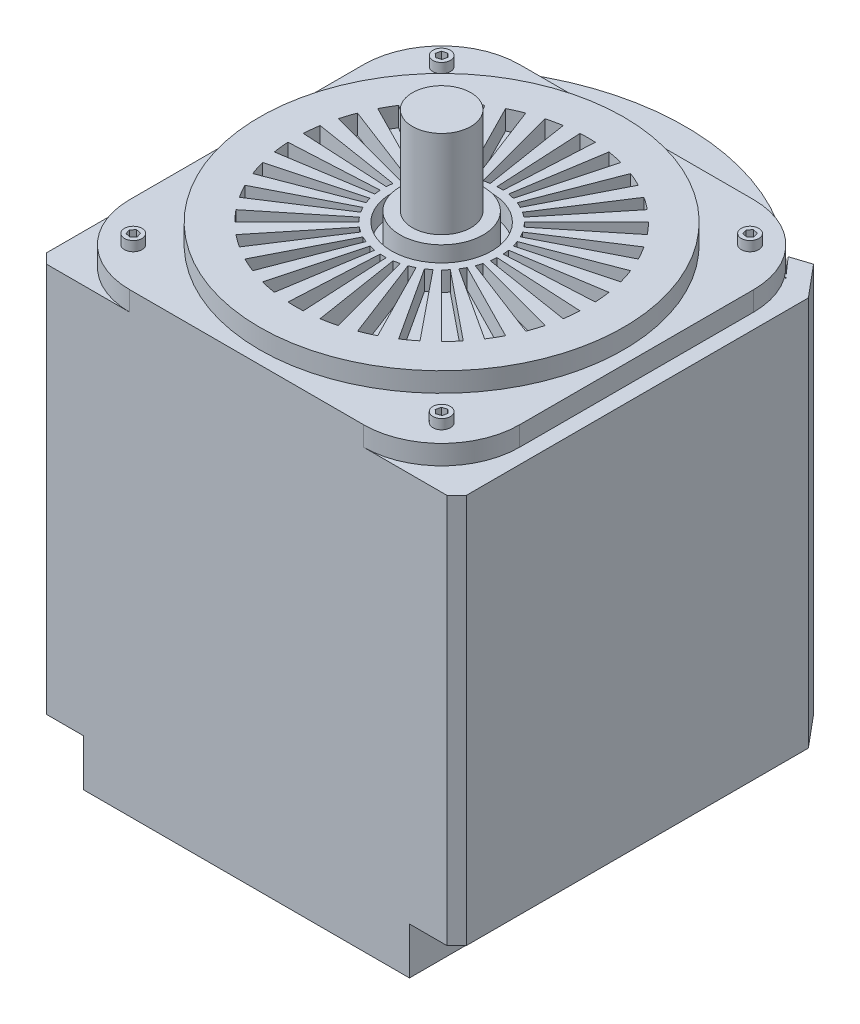
from build123d import *

# Parameters (mm, degrees)
BOSS_EXTRUDE1_DEPTH  = 200
BOSS_EXTRUDE2_DEPTH  = 200
BOSS_EXTRUDE5_DEPTH  = 10
SKETCH4_W            = 215.39447181
SKETCH4_H            = 200
BOSS_EXTRUDE6_DEPTH  = 17.479413836
BOSS_EXTRUDE7_START  = -30
BOSS_EXTRUDE7_DEPTH  = 30
SKETCH6_R            = 93.394786631
SKETCH6_R_2          = 25.673821091
BOSS_EXTRUDE8_DEPTH  = 10
SKETCH7_R            = 21.331945156
BOSS_EXTRUDE9_DEPTH  = 15
SKETCH8_R            = 15
BOSS_EXTRUDE10_DEPTH = 45
SKETCH9_R            = 4.5
BOSS_EXTRUDE11_DEPTH = 5
CUT_EXTRUDE1_DEPTH   = 4
CIRPATTERN1_COUNT    = 4
BOSS_EXTRUDE12_DEPTH = 4
BOSS_EXTRUDE13_DEPTH = 24
CHAMFER1_SIZE        = 5
SKETCH13_R           = 6.5
CUT_EXTRUDE2_DEPTH   = 30
SKETCH14_R           = 5.5
BOSS_EXTRUDE14_DEPTH = 4


with BuildPart() as part:
    # Sketch1 → Boss-Extrude1 (new body)
    with BuildSketch(Plane(origin=(0, 0, 0), x_dir=(1, 0, 0), z_dir=(0, 1, 0))):
        with BuildLine():
            Line((-1.5, 124.990999676), (-5.554426032, 109.85967573))
            ThreePointArc((-5.554426032, 109.85967573), (-7.673212112, 109.732045529), (-9.789141002, 109.563555612))
            Line((-9.789141002, 109.563555612), (-15.909982914, 123.983355511))
            ThreePointArc((-15.909982914, 123.983355511), (-17.39663762, 123.783508593), (-18.88078712, 123.565836208))
            Line((-18.88078712, 123.565836208), (-20.789882481, 108.017502223))
            ThreePointArc((-20.789882481, 108.017502223), (-22.87028599, 107.596236081), (-24.942173542, 107.134905512))
            Line((-24.942173542, 107.134905512), (-33.010296108, 120.562516359))
            ThreePointArc((-33.010296108, 120.562516359), (-34.454669477, 120.157711992), (-35.894081196, 119.735604292))
            Line((-35.894081196, 119.735604292), (-35.620687516, 104.072890903))
            ThreePointArc((-35.620687516, 104.072890903), (-37.622215766, 103.366188286), (-39.609735045, 102.620996339))
            Line((-39.609735045, 102.620996339), (-49.468101436, 114.795064965))
            ThreePointArc((-49.468101436, 114.795064965), (-50.842080384, 114.193182205), (-52.208737809, 113.574855036))
            Line((-52.208737809, 113.574855036), (-49.758176387, 98.102619143))
            ThreePointArc((-49.758176387, 98.102619143), (-51.641871906, 97.124235214), (-53.50633811, 96.109686203))
            Line((-53.50633811, 96.109686203), (-64.96306644, 106.793258208))
            ThreePointArc((-64.96306644, 106.793258208), (-66.239908029, 106.00601202), (-67.507210728, 105.203500416))
            Line((-67.507210728, 105.203500416), (-62.927178953, 90.222891491))
            ThreePointArc((-62.927178953, 90.222891491), (-64.656377752, 88.991869381), (-66.361501167, 87.727710348))
            Line((-66.361501167, 87.727710348), (-79.193599249, 96.712842156))
            ThreePointArc((-79.193599249, 96.712842156), (-80.348451211, 95.75555539), (-81.491732579, 94.784479327))
            Line((-81.491732579, 94.784479327), (-74.87137556, 80.587077884))
            ThreePointArc((-74.87137556, 80.587077884), (-76.41242075, 79.127378037), (-77.925013089, 77.638214399))
            Line((-77.925013089, 77.638214399), (-91.882718731, 84.750020641))
            ThreePointArc((-91.882718731, 84.750020641), (-92.893103185, 83.641325795), (-93.89011055, 82.520586164))
            Line((-93.89011055, 82.520586164), (-93.89011055, -82.520586164))
            Line((-93.89011055, -82.520586164), (93.697235905, -82.520586164))
            Line((93.697235905, -82.520586164), (93.697235905, 82.739518876))
            ThreePointArc((93.697235905, 82.739518876), (92.697615235, 83.857928247), (91.684645627, 84.964261641))
            Line((91.684645627, 84.964261641), (77.743578328, 77.819894814))
            ThreePointArc((77.743578328, 77.819894814), (76.24293888, 79.290694731), (74.714479133, 80.732562253))
            Line((74.714479133, 80.732562253), (81.307207406, 94.942814493))
            ThreePointArc((81.307207406, 94.942814493), (80.162039302, 95.911664853), (79.005327449, 96.866703436))
            Line((79.005327449, 96.866703436), (66.190731164, 87.856628139))
            ThreePointArc((66.190731164, 87.856628139), (64.50048555, 89.104923342), (62.786704343, 90.320705034))
            Line((62.786704343, 90.320705034), (67.343418819, 105.308422939))
            ThreePointArc((67.343418819, 105.308422939), (66.074868843, 106.108961485), (64.796803743, 106.894219791))
            Line((64.796803743, 106.894219791), (53.356714297, 96.192832578))
            ThreePointArc((53.356714297, 96.192832578), (51.509578449, 97.194461406), (49.643647261, 98.16062493))
            Line((49.643647261, 98.16062493), (52.07614942, 113.635710327))
            ThreePointArc((52.07614942, 113.635710327), (50.708771279, 114.252442054), (49.334090811, 114.852720838))
            Line((49.334090811, 114.852720838), (39.489939448, 102.667154837))
            ThreePointArc((39.489939448, 102.667154837), (37.521666022, 103.402730036), (35.53970131, 104.100574594))
            Line((35.53970131, 104.100574594), (35.800908304, 119.76349596))
            ThreePointArc((35.800908304, 119.76349596), (34.361168595, 120.184483578), (32.916480699, 120.588164006))
            Line((32.916480699, 120.588164006), (24.858808122, 107.154279703))
            ThreePointArc((24.858808122, 107.154279703), (22.807494482, 107.60956368), (20.747858611, 108.025581984))
            Line((20.747858611, 108.025581984), (18.832714591, 123.573172093))
            ThreePointArc((18.832714591, 123.573172093), (17.348480521, 123.790267079), (15.861748181, 123.989535626))
            Line((15.861748181, 123.989535626), (9.7465165, 109.567355613))
            ThreePointArc((9.7465165, 109.567355613), (7.651867312, 109.733536016), (5.554426032, 109.85967573))
            Line((5.554426032, 109.85967573), (1.5, 124.990999676))
            ThreePointArc((1.5, 124.990999676), (0, 125), (-1.5, 124.990999676))
        make_face()
    extrude(amount=BOSS_EXTRUDE1_DEPTH)

    # Sketch2 → Boss-Extrude2 (add)
    with BuildSketch(Plane(origin=(0, 200, 0), x_dir=(1, 0, 0), z_dir=(0, 1, 0))):
        Polygon((-93.89011055, 82.520586164), (-84.247016889, 93.492286342), (-94.044433488, 96.7026075), (-107.697235905, 80.401462252), (-107.697235905, -82.520586164), (-93.89011055, -82.520586164), align=None)
        Polygon((93.697235905, 82.739518876), (93.697235905, -82.520586164), (107.697235905, -82.520586164), (107.697235905, 80.401462252), (94.044433488, 96.7026075), (84.247016889, 93.492286342), align=None)
    extrude(amount=-BOSS_EXTRUDE2_DEPTH)

    # Sketch3 → Boss-Extrude5 (add)
    with BuildSketch(Plane(origin=(0, 200, 0), x_dir=(1, 0, 0), z_dir=(0, 1, 0))):
        with BuildLine():
            Line((-60, -100), (60, -100))
            ThreePointArc((60, -100), (88.284271247, -88.284271247), (100, -60))
            Line((100, -60), (100, 60))
            ThreePointArc((100, 60), (88.284271247, 88.284271247), (60, 100))
            Line((60, 100), (-60, 100))
            ThreePointArc((-60, 100), (-88.284271247, 88.284271247), (-100, 60))
            Line((-100, 60), (-100, -60))
            ThreePointArc((-100, -60), (-88.284271247, -88.284271247), (-60, -100))
        make_face()
    extrude(amount=BOSS_EXTRUDE5_DEPTH)

    # Sketch4 → Boss-Extrude6 (add)
    with BuildSketch(Plane.XY.offset(82.520586164)):
        with Locations((0, 100)):
            Rectangle(SKETCH4_W, SKETCH4_H)
    extrude(amount=BOSS_EXTRUDE6_DEPTH)

    # Sketch5 → Boss-Extrude7 (add)
    with BuildSketch(Plane(origin=(0, 200, 0), x_dir=(1, 0, 0), z_dir=(0, 1, 0)).offset(BOSS_EXTRUDE7_START)):
        with BuildLine():
            Line((-102.459320776, 71.603684167), (0, 0))
            Line((0, 0), (95.193765048, 81.013252595))
            ThreePointArc((95.193765048, 81.013252595), (-5.944078525, 124.858591737), (-102.459320776, 71.603684167))
        make_face()
    boss_extrude7 = extrude(amount=BOSS_EXTRUDE7_DEPTH)

    # Mirror2: Boss-Extrude7 across plane
    add(boss_extrude7.mirror(Plane(origin=(0, 100, 0), x_dir=(0, 0, 1), z_dir=(0, -1, 0))))

    # Sketch6 → Boss-Extrude8 (add)
    with BuildSketch(Plane(origin=(0, 210, 0), x_dir=(1, 0, 0), z_dir=(0, 1, 0))):
        with Locations(Location((0, 0, 0), (0, 0, 270))):
            Circle(SKETCH6_R)
        with Locations(Location((0, 0, 0), (0, 0, 270))):
            Circle(SKETCH6_R_2, mode=Mode.SUBTRACT)
        with BuildLine():
            Line((-3.925196718, 74.897215107), (-1.570078687, 29.958886043))
            ThreePointArc((-1.570078687, 29.958886043), (0, 30), (1.570078687, 29.958886043))
            Line((1.570078687, 29.958886043), (3.925196718, 74.897215107))
            ThreePointArc((3.925196718, 74.897215107), (0, 75), (-3.925196718, 74.897215107))
        make_face(mode=Mode.SUBTRACT)
        with BuildLine():
            Line((11.732584878, 74.076625545), (4.693033951, 29.630650218))
            ThreePointArc((4.693033951, 29.630650218), (6.237350725, 29.344428022), (7.764571353, 28.977774789))
            Line((7.764571353, 28.977774789), (19.411428383, 72.444436972))
            ThreePointArc((19.411428383, 72.444436972), (15.593376811, 73.361070055), (11.732584878, 74.076625545))
        make_face(mode=Mode.SUBTRACT)
        with BuildLine():
            Line((26.877596216, 70.018531987), (10.751038486, 28.007412795))
            ThreePointArc((10.751038486, 28.007412795), (12.202099292, 27.406363729), (13.619714992, 26.730195726))
            Line((13.619714992, 26.730195726), (34.04928748, 66.825489314))
            ThreePointArc((34.04928748, 66.825489314), (30.505248231, 68.515909323), (26.877596216, 70.018531987))
        make_face(mode=Mode.SUBTRACT)
        with BuildLine():
            Line((40.847927626, 62.900292596), (16.33917105, 25.160117038))
            ThreePointArc((16.33917105, 25.160117038), (17.633557569, 24.270509831), (18.879611731, 23.314378844))
            Line((18.879611731, 23.314378844), (47.199029329, 58.285947109))
            ThreePointArc((47.199029329, 58.285947109), (44.083893922, 60.676274578), (40.847927626, 62.900292596))
        make_face(mode=Mode.SUBTRACT)
        with BuildLine():
            Line((53.033008589, 53.033008589), (21.213203436, 21.213203436))
            ThreePointArc((21.213203436, 21.213203436), (22.294344764, 20.073918191), (23.314378844, 18.879611731))
            Line((23.314378844, 18.879611731), (58.285947109, 47.199029329))
            ThreePointArc((58.285947109, 47.199029329), (55.735861911, 50.184795477), (53.033008589, 53.033008589))
        make_face(mode=Mode.SUBTRACT)
        with BuildLine():
            Line((62.900292596, 40.847927626), (25.160117038, 16.33917105))
            ThreePointArc((25.160117038, 16.33917105), (25.980762114, 15), (26.730195726, 13.619714992))
            Line((26.730195726, 13.619714992), (66.825489314, 34.04928748))
            ThreePointArc((66.825489314, 34.04928748), (64.951905284, 37.5), (62.900292596, 40.847927626))
        make_face(mode=Mode.SUBTRACT)
        with BuildLine():
            Line((70.018531987, 26.877596216), (28.007412795, 10.751038486))
            ThreePointArc((28.007412795, 10.751038486), (28.531695489, 9.270509831), (28.977774789, 7.764571353))
            Line((28.977774789, 7.764571353), (72.444436972, 19.411428383))
            ThreePointArc((72.444436972, 19.411428383), (71.329238722, 23.176274578), (70.018531987, 26.877596216))
        make_face(mode=Mode.SUBTRACT)
        with BuildLine():
            Line((74.076625545, 11.732584878), (29.630650218, 4.693033951))
            ThreePointArc((29.630650218, 4.693033951), (29.835656861, 3.135853898), (29.958886043, 1.570078687))
            Line((29.958886043, 1.570078687), (74.897215107, 3.925196718))
            ThreePointArc((74.897215107, 3.925196718), (74.589142153, 7.839634745), (74.076625545, 11.732584878))
        make_face(mode=Mode.SUBTRACT)
        with BuildLine():
            Line((74.897215107, -3.925196718), (29.958886043, -1.570078687))
            ThreePointArc((29.958886043, -1.570078687), (29.835656861, -3.135853898), (29.630650218, -4.693033951))
            Line((29.630650218, -4.693033951), (74.076625545, -11.732584878))
            ThreePointArc((74.076625545, -11.732584878), (74.589142153, -7.839634745), (74.897215107, -3.925196718))
        make_face(mode=Mode.SUBTRACT)
        with BuildLine():
            Line((72.444436972, -19.411428383), (28.977774789, -7.764571353))
            ThreePointArc((28.977774789, -7.764571353), (28.531695489, -9.270509831), (28.007412795, -10.751038486))
            Line((28.007412795, -10.751038486), (70.018531987, -26.877596216))
            ThreePointArc((70.018531987, -26.877596216), (71.329238722, -23.176274578), (72.444436972, -19.411428383))
        make_face(mode=Mode.SUBTRACT)
        with BuildLine():
            Line((66.825489314, -34.04928748), (26.730195726, -13.619714992))
            ThreePointArc((26.730195726, -13.619714992), (25.980762114, -15), (25.160117038, -16.33917105))
            Line((25.160117038, -16.33917105), (62.900292596, -40.847927626))
            ThreePointArc((62.900292596, -40.847927626), (64.951905284, -37.5), (66.825489314, -34.04928748))
        make_face(mode=Mode.SUBTRACT)
        with BuildLine():
            Line((58.285947109, -47.199029329), (23.314378844, -18.879611731))
            ThreePointArc((23.314378844, -18.879611731), (22.294344764, -20.073918191), (21.213203436, -21.213203436))
            Line((21.213203436, -21.213203436), (53.033008589, -53.033008589))
            ThreePointArc((53.033008589, -53.033008589), (55.735861911, -50.184795477), (58.285947109, -47.199029329))
        make_face(mode=Mode.SUBTRACT)
        with BuildLine():
            Line((47.199029329, -58.285947109), (18.879611731, -23.314378844))
            ThreePointArc((18.879611731, -23.314378844), (17.633557569, -24.270509831), (16.33917105, -25.160117038))
            Line((16.33917105, -25.160117038), (40.847927626, -62.900292596))
            ThreePointArc((40.847927626, -62.900292596), (44.083893922, -60.676274578), (47.199029329, -58.285947109))
        make_face(mode=Mode.SUBTRACT)
        with BuildLine():
            Line((34.04928748, -66.825489314), (13.619714992, -26.730195726))
            ThreePointArc((13.619714992, -26.730195726), (12.202099292, -27.406363729), (10.751038486, -28.007412795))
            Line((10.751038486, -28.007412795), (26.877596216, -70.018531987))
            ThreePointArc((26.877596216, -70.018531987), (30.505248231, -68.515909323), (34.04928748, -66.825489314))
        make_face(mode=Mode.SUBTRACT)
        with BuildLine():
            Line((19.411428383, -72.444436972), (7.764571353, -28.977774789))
            ThreePointArc((7.764571353, -28.977774789), (6.237350725, -29.344428022), (4.693033951, -29.630650218))
            Line((4.693033951, -29.630650218), (11.732584878, -74.076625545))
            ThreePointArc((11.732584878, -74.076625545), (15.593376811, -73.361070055), (19.411428383, -72.444436972))
        make_face(mode=Mode.SUBTRACT)
        with BuildLine():
            Line((3.925196718, -74.897215107), (1.570078687, -29.958886043))
            ThreePointArc((1.570078687, -29.958886043), (0, -30), (-1.570078687, -29.958886043))
            Line((-1.570078687, -29.958886043), (-3.925196718, -74.897215107))
            ThreePointArc((-3.925196718, -74.897215107), (0, -75), (3.925196718, -74.897215107))
        make_face(mode=Mode.SUBTRACT)
        with BuildLine():
            Line((-11.732584878, -74.076625545), (-4.693033951, -29.630650218))
            ThreePointArc((-4.693033951, -29.630650218), (-6.237350725, -29.344428022), (-7.764571353, -28.977774789))
            Line((-7.764571353, -28.977774789), (-19.411428383, -72.444436972))
            ThreePointArc((-19.411428383, -72.444436972), (-15.593376811, -73.361070055), (-11.732584878, -74.076625545))
        make_face(mode=Mode.SUBTRACT)
        with BuildLine():
            Line((-26.877596216, -70.018531987), (-10.751038486, -28.007412795))
            ThreePointArc((-10.751038486, -28.007412795), (-12.202099292, -27.406363729), (-13.619714992, -26.730195726))
            Line((-13.619714992, -26.730195726), (-34.04928748, -66.825489314))
            ThreePointArc((-34.04928748, -66.825489314), (-30.505248231, -68.515909323), (-26.877596216, -70.018531987))
        make_face(mode=Mode.SUBTRACT)
        with BuildLine():
            Line((-40.847927626, -62.900292596), (-16.33917105, -25.160117038))
            ThreePointArc((-16.33917105, -25.160117038), (-17.633557569, -24.270509831), (-18.879611731, -23.314378844))
            Line((-18.879611731, -23.314378844), (-47.199029329, -58.285947109))
            ThreePointArc((-47.199029329, -58.285947109), (-44.083893922, -60.676274578), (-40.847927626, -62.900292596))
        make_face(mode=Mode.SUBTRACT)
        with BuildLine():
            Line((-53.033008589, -53.033008589), (-21.213203436, -21.213203436))
            ThreePointArc((-21.213203436, -21.213203436), (-22.294344764, -20.073918191), (-23.314378844, -18.879611731))
            Line((-23.314378844, -18.879611731), (-58.285947109, -47.199029329))
            ThreePointArc((-58.285947109, -47.199029329), (-55.735861911, -50.184795477), (-53.033008589, -53.033008589))
        make_face(mode=Mode.SUBTRACT)
        with BuildLine():
            Line((-62.900292596, -40.847927626), (-25.160117038, -16.33917105))
            ThreePointArc((-25.160117038, -16.33917105), (-25.980762114, -15), (-26.730195726, -13.619714992))
            Line((-26.730195726, -13.619714992), (-66.825489314, -34.04928748))
            ThreePointArc((-66.825489314, -34.04928748), (-64.951905284, -37.5), (-62.900292596, -40.847927626))
        make_face(mode=Mode.SUBTRACT)
        with BuildLine():
            Line((-70.018531987, -26.877596216), (-28.007412795, -10.751038486))
            ThreePointArc((-28.007412795, -10.751038486), (-28.531695489, -9.270509831), (-28.977774789, -7.764571353))
            Line((-28.977774789, -7.764571353), (-72.444436972, -19.411428383))
            ThreePointArc((-72.444436972, -19.411428383), (-71.329238722, -23.176274578), (-70.018531987, -26.877596216))
        make_face(mode=Mode.SUBTRACT)
        with BuildLine():
            Line((-74.076625545, -11.732584878), (-29.630650218, -4.693033951))
            ThreePointArc((-29.630650218, -4.693033951), (-29.835656861, -3.135853898), (-29.958886043, -1.570078687))
            Line((-29.958886043, -1.570078687), (-74.897215107, -3.925196718))
            ThreePointArc((-74.897215107, -3.925196718), (-74.589142153, -7.839634745), (-74.076625545, -11.732584878))
        make_face(mode=Mode.SUBTRACT)
        with BuildLine():
            Line((-74.897215107, 3.925196718), (-29.958886043, 1.570078687))
            ThreePointArc((-29.958886043, 1.570078687), (-29.835656861, 3.135853898), (-29.630650218, 4.693033951))
            Line((-29.630650218, 4.693033951), (-74.076625545, 11.732584878))
            ThreePointArc((-74.076625545, 11.732584878), (-74.589142153, 7.839634745), (-74.897215107, 3.925196718))
        make_face(mode=Mode.SUBTRACT)
        with BuildLine():
            Line((-72.444436972, 19.411428383), (-28.977774789, 7.764571353))
            ThreePointArc((-28.977774789, 7.764571353), (-28.531695489, 9.270509831), (-28.007412795, 10.751038486))
            Line((-28.007412795, 10.751038486), (-70.018531987, 26.877596216))
            ThreePointArc((-70.018531987, 26.877596216), (-71.329238722, 23.176274578), (-72.444436972, 19.411428383))
        make_face(mode=Mode.SUBTRACT)
        with BuildLine():
            Line((-66.825489314, 34.04928748), (-26.730195726, 13.619714992))
            ThreePointArc((-26.730195726, 13.619714992), (-25.980762114, 15), (-25.160117038, 16.33917105))
            Line((-25.160117038, 16.33917105), (-62.900292596, 40.847927626))
            ThreePointArc((-62.900292596, 40.847927626), (-64.951905284, 37.5), (-66.825489314, 34.04928748))
        make_face(mode=Mode.SUBTRACT)
        with BuildLine():
            Line((-58.285947109, 47.199029329), (-23.314378844, 18.879611731))
            ThreePointArc((-23.314378844, 18.879611731), (-22.294344764, 20.073918191), (-21.213203436, 21.213203436))
            Line((-21.213203436, 21.213203436), (-53.033008589, 53.033008589))
            ThreePointArc((-53.033008589, 53.033008589), (-55.735861911, 50.184795477), (-58.285947109, 47.199029329))
        make_face(mode=Mode.SUBTRACT)
        with BuildLine():
            Line((-47.199029329, 58.285947109), (-18.879611731, 23.314378844))
            ThreePointArc((-18.879611731, 23.314378844), (-17.633557569, 24.270509831), (-16.33917105, 25.160117038))
            Line((-16.33917105, 25.160117038), (-40.847927626, 62.900292596))
            ThreePointArc((-40.847927626, 62.900292596), (-44.083893922, 60.676274578), (-47.199029329, 58.285947109))
        make_face(mode=Mode.SUBTRACT)
        with BuildLine():
            Line((-34.04928748, 66.825489314), (-13.619714992, 26.730195726))
            ThreePointArc((-13.619714992, 26.730195726), (-12.202099292, 27.406363729), (-10.751038486, 28.007412795))
            Line((-10.751038486, 28.007412795), (-26.877596216, 70.018531987))
            ThreePointArc((-26.877596216, 70.018531987), (-30.505248231, 68.515909323), (-34.04928748, 66.825489314))
        make_face(mode=Mode.SUBTRACT)
        with BuildLine():
            Line((-19.411428383, 72.444436972), (-7.764571353, 28.977774789))
            ThreePointArc((-7.764571353, 28.977774789), (-6.237350725, 29.344428022), (-4.693033951, 29.630650218))
            Line((-4.693033951, 29.630650218), (-11.732584878, 74.076625545))
            ThreePointArc((-11.732584878, 74.076625545), (-15.593376811, 73.361070055), (-19.411428383, 72.444436972))
        make_face(mode=Mode.SUBTRACT)
    extrude(amount=BOSS_EXTRUDE8_DEPTH)

    # Sketch7 → Boss-Extrude9 (add)
    with BuildSketch(Plane(origin=(0, 210, 0), x_dir=(1, 0, 0), z_dir=(0, 1, 0))):
        with Locations(Location((0, 0, 0), (0, 0, 270))):
            Circle(SKETCH7_R)
    extrude(amount=BOSS_EXTRUDE9_DEPTH)

    # Sketch8 → Boss-Extrude10 (add)
    with BuildSketch(Plane(origin=(0, 225, 0), x_dir=(1, 0, 0), z_dir=(0, 1, 0))):
        with Locations(Location((0, 0, 0), (0, 0, 90))):
            Circle(SKETCH8_R)
    extrude(amount=BOSS_EXTRUDE10_DEPTH)

    # Sketch9 → Boss-Extrude11 (add)
    with BuildSketch(Plane(origin=(0, 210, 0), x_dir=(1, 0, 0), z_dir=(0, 1, 0))):
        with Locations(Location((-79.091883092, 79.091883092, 0), (0, 0, 270))):
            Circle(SKETCH9_R)
    boss_extrude11 = extrude(amount=BOSS_EXTRUDE11_DEPTH)

    # Sketch10 → Cut-Extrude1 (cut)
    with BuildSketch(Plane(origin=(0, 215, 0), x_dir=(1, 0, 0), z_dir=(0, 1, 0))):
        Polygon((-77.136997259, 77.338057827), (-76.595582942, 79.907951253), (-78.550468775, 81.661776518), (-81.046768926, 80.845708357), (-81.588183242, 78.275814931), (-79.633297409, 76.521989666), align=None)
    cut_extrude1 = extrude(amount=-CUT_EXTRUDE1_DEPTH, mode=Mode.SUBTRACT)

    # CirPattern1: Boss-Extrude11, Cut-Extrude1 ×4 about axis
    cirpattern1_axis = Axis((0, 0, 0), (0, 1, 0))
    add([boss_extrude11.rotate(cirpattern1_axis, i * 360 / CIRPATTERN1_COUNT) for i in range(1, CIRPATTERN1_COUNT)])
    add([cut_extrude1.rotate(cirpattern1_axis, i * 360 / CIRPATTERN1_COUNT) for i in range(1, CIRPATTERN1_COUNT)], mode=Mode.SUBTRACT)

    # Sketch11 → Boss-Extrude12 (add)
    with BuildSketch(Plane.XZ):
        Polygon((-84.247016889, -93.492286342), (-80.973407917, -90.218677371), (-95.934039507, -80.850186969), align=None)
        Polygon((84.247016889, -93.492286342), (80.641453694, -91.234448231), (99.062645219, -78.291639573), align=None)
    extrude(amount=-BOSS_EXTRUDE12_DEPTH)

    # Sketch12 → Boss-Extrude13 (add)
    with BuildSketch(Plane.XZ):
        with BuildLine():
            Line((-83.644750236, -92.89001969), (-83.644750236, 100))
            Line((-83.644750236, 100), (83.497153156, 100))
            Line((83.497153156, 100), (83.497153156, -93.02271451))
            ThreePointArc((83.497153156, -93.02271451), (-0.099238115, -124.999960607), (-83.644750236, -92.89001969))
        make_face()
    extrude(amount=BOSS_EXTRUDE13_DEPTH)

    # Chamfer1
    chamfer1_edges = [part.edges().sort_by_distance(p)[0] for p in [
        (107.697235905, 100, 100),
        (-107.697235905, 100, 100),
    ]]
    chamfer(chamfer1_edges, length=CHAMFER1_SIZE)

    # Sketch13 → Cut-Extrude2 (cut)
    with BuildSketch(Plane(origin=(0, 0, -125), x_dir=(-1, 0, 0), z_dir=(0, 0, -1))):
        with Locations(Location((-68.497153156, 185, 0), (0, 0, 90))):
            Circle(SKETCH13_R)
        with Locations(Location((68.644750236, 185, 0), (0, 0, 90))):
            Circle(SKETCH13_R)
        with Locations(Location((-68.497153156, -9, 0), (0, 0, 90))):
            Circle(SKETCH13_R)
        with Locations(Location((68.644750236, -9, 0), (0, 0, 90))):
            Circle(SKETCH13_R)
    extrude(amount=-CUT_EXTRUDE2_DEPTH, mode=Mode.SUBTRACT)

    # Sketch14 → Boss-Extrude14 (add)
    # profile 1 of 4: a face of its own
    with BuildSketch(Plane(origin=(0, 0, -95), x_dir=(-1, 0, 0), z_dir=(0, 0, -1))):
        with Locations(Location((-68.497153156, 185, 0), (0, 0, 90))):
            Circle(SKETCH14_R)
        Polygon((-65.711252358, 183.128826371), (-65.483718859, 186.477074049), (-68.269619657, 188.348247678), (-71.283053953, 186.871173629), (-71.510587452, 183.522925951), (-68.724686655, 181.651752322), align=None, mode=Mode.SUBTRACT)
    # profile 2 of 4: a face of its own
    with BuildSketch(Plane(origin=(0, 0, -95), x_dir=(-1, 0, 0), z_dir=(0, 0, -1))):
        with Locations(Location((68.644750236, 185, 0), (0, 0, 90))):
            Circle(SKETCH14_R)
        Polygon((69.743373926, 181.651752322), (72.093729628, 184.277312186), (70.995105938, 187.625559864), (67.546126546, 188.348247678), (65.195770844, 185.722687814), (66.294394534, 182.374440136), align=None, mode=Mode.SUBTRACT)
    # profile 3 of 4: a face of its own
    with BuildSketch(Plane(origin=(0, 0, -95), x_dir=(-1, 0, 0), z_dir=(0, 0, -1))):
        with Locations(Location((-68.497153156, -9, 0), (0, 0, 90))):
            Circle(SKETCH14_R)
        Polygon((-71.689082014, -9.415543774), (-69.73324612, -11.972063365), (-66.541317262, -11.556519591), (-65.305224297, -8.584456226), (-67.261060191, -6.027936635), (-70.45298905, -6.443480409), align=None, mode=Mode.SUBTRACT)
    # profile 4 of 4: a face of its own
    with BuildSketch(Plane(origin=(0, 0, -95), x_dir=(-1, 0, 0), z_dir=(0, 0, -1))):
        with Locations(Location((68.644750236, -9, 0), (0, 0, 90))):
            Circle(SKETCH14_R)
        Polygon((70.893631359, -11.048950365), (71.543633865, -8.076887), (69.294752742, -6.027936635), (66.395869113, -6.951049635), (65.745866607, -9.923113), (67.99474773, -11.972063365), align=None, mode=Mode.SUBTRACT)
    extrude(amount=BOSS_EXTRUDE14_DEPTH)


solid = part.part
